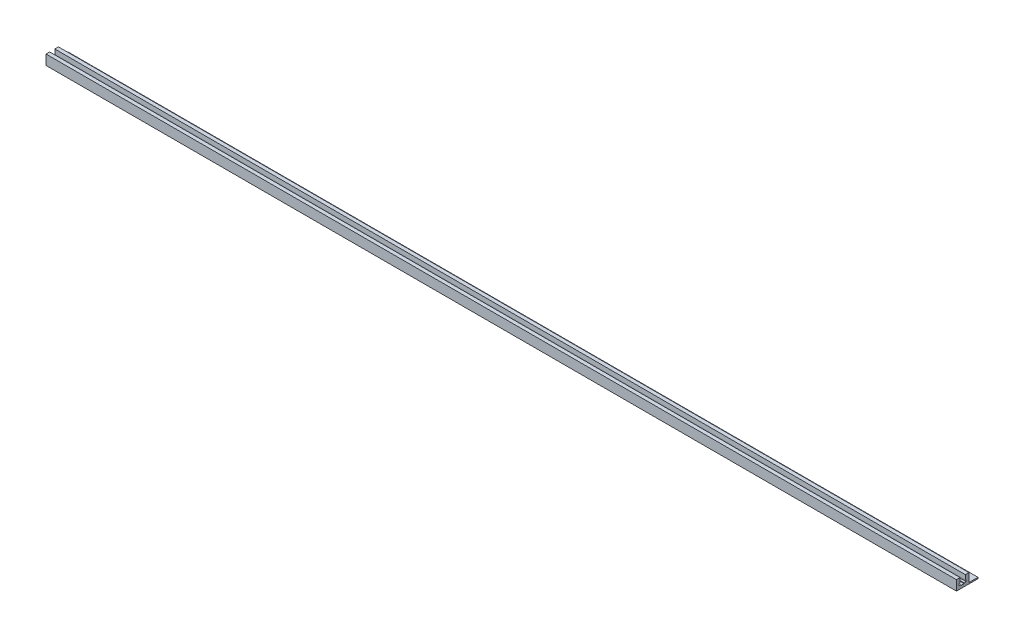
SolidWorks part; units mm, degrees
ref_plane "前视基准面" through (0, 0, 0) normal (0, 0, 1) x (1, 0, 0)
ref_plane "上视基准面" through (0, 0, 0) normal (0, 1, 0) x (1, 0, 0)
ref_plane "右视基准面" through (0, 0, 0) normal (1, 0, 0) x (0, 0, -1)
sketch "草图1" plane through (0, 0, 0) normal (1, 0, 0) x (0, 0, -1)
  line L1 (-15, 12) -> (15, 12)
  line L2 (-15, 12) -> (-15, -12)
  line L3 (-15, -12) -> (15, -12)
  line L4 (15, 12) -> (15, -12)
  line L5 (-15, 12) -> (15, -12) construction
  line L6 (-15, -12) -> (15, 12) construction
  point P0 (0, 0)
  dimension "D1" = 30
  dimension "D2" = 24
extrude "凸台-拉伸1" add sketch "草图1" along normal blind 2200
sketch "草图2" plane through (2200, 0, 0) normal (1, 0, 0) x (0, 0, -1)
  line L0 (-6.2, 12) -> (-6.2, 0.7)
  line L1 (15, 12) -> (-15, 12) construction
  line L2 (-6.2, 0.7) -> (-8.5, 0.7)
  line L3 (-8.5, 0.7) -> (-8.5, -3.9)
  line L4 (-8.5, -3.9) -> (-3.5, -3.9)
  line L5 (-3.5, -3.9) -> (-3.5, -5.5)
  line L6 (-3.5, -5.5) -> (3.5, -5.5)
  line L7 (0, -5.5) -> (0, 14.908) construction
  line L8 (3.5, -3.9) -> (3.5, -5.5)
  line L9 (8.5, -3.9) -> (3.5, -3.9)
  line L10 (8.5, 0.7) -> (8.5, -3.9)
  line L11 (6.2, 0.7) -> (8.5, 0.7)
  line L12 (6.2, 12) -> (6.2, 0.7)
  line L13 (-6.2, 12) -> (6.2, 12)
  dimension "D1" = 12.4
  dimension "D2" = 7
  dimension "D3" = 17
  dimension "D4" = 11.3
  dimension "D5" = 15.9
  dimension "D6" = 17.5
extrude "切除-拉伸1" cut sketch "草图2" against normal through all contours L12 L11 L10 L9 L8 L6 L5 L4 L3 L2 L0 L13
sketch "草图5" plane through (0, 0, -15) normal (0, 0, -1) x (-1, 0, 0)
  line L1 (-2200, -12) -> (0, -12)
  line L2 (-2200, -12) -> (-2200, -9)
  line L3 (-2200, -9) -> (0, -9)
  line L4 (0, -12) -> (0, -9)
  dimension "D1" = 3
extrude "凸台-拉伸2" add sketch "草图5" along normal blind 22
sketch "草图6" plane through (0, -12, 0) normal (0, -1, 0) x (1, 0, 0)
  line L0 (30, -22) -> (30, -30) construction
  line L1 (33.5, -22) -> (33.5, -30)
  line L2 (26.5, -22) -> (26.5, -30)
  line L3 (2200, -37) -> (0, -37) construction
  line L4 (0, 15) -> (0, -37) construction
  arc A0 (33.5, -22) -> (26.5, -22) centre (30, -22) ccw
  arc A1 (26.5, -30) -> (33.5, -30) centre (30, -30) ccw
  point P2 (30, -26)
  dimension "D1" = 7
  dimension "D2" = 8
  dimension "D3" = 11
  dimension "D4" = 30
extrude "切除-拉伸2" cut sketch "草图6" against normal blind 22
pattern_linear "阵列(线性)1" count 6 spacing 510 along (1, 0, 0) of "切除-拉伸2"
